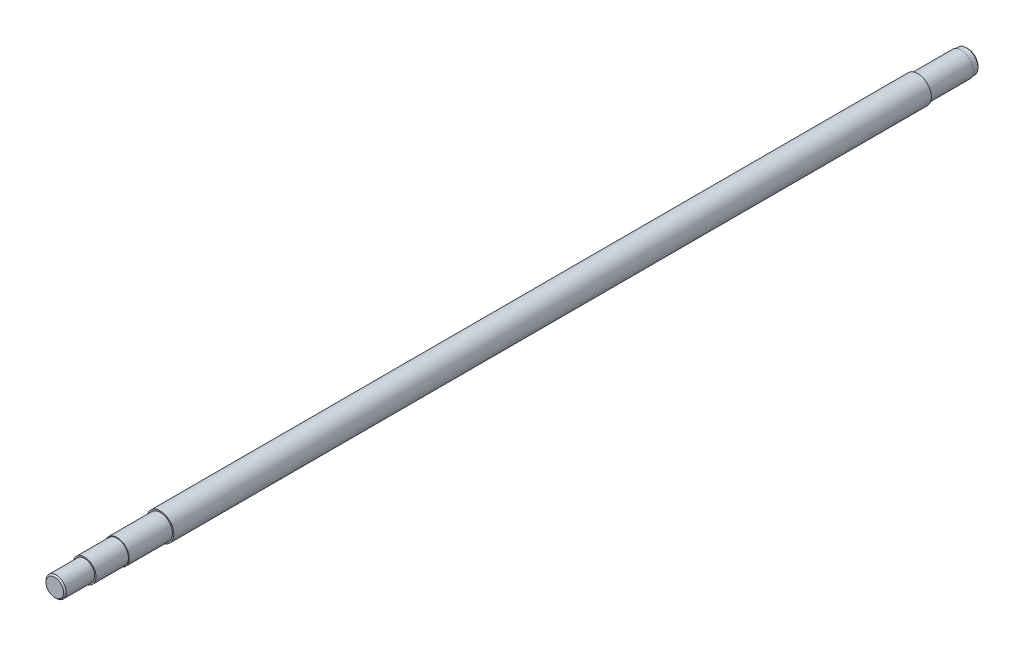
SolidWorks part; units mm, degrees
ref_plane "前视基准面" through (0, 0, 0) normal (0, 0, 1) x (1, 0, 0)
ref_plane "上视基准面" through (0, 0, 0) normal (0, 1, 0) x (1, 0, 0)
ref_plane "右视基准面" through (0, 0, 0) normal (1, 0, 0) x (0, 0, -1)
other "Configuration Table"
sketch "草图1" plane through (0, 0, 0) normal (0, 0, 1) x (1, 0, 0)
  circle A0 centre (0, 0) radius 37.5
  dimension "D1" = 75
extrude "凸台-拉伸1" add sketch "草图1" along normal blind 140 contours A0
sketch "草图2" plane through (0, 0, 140) normal (0, 0, 1) x (1, 0, 0)
  circle A0 centre (0, 0) radius 42.5
  dimension "D1" = 85
extrude "凸台-拉伸2" add sketch "草图2" along normal blind 120 contours A0
sketch "草图3" plane through (0, 0, 260) normal (0, 0, 1) x (1, 0, 0)
  circle A0 centre (0, 0) radius 45
  dimension "D1" = 90
extrude "凸台-拉伸3" add sketch "草图3" along normal blind 160 contours A0
sketch "草图4" plane through (0, 0, 420) normal (0, 0, 1) x (1, 0, 0)
  circle A0 centre (0, 0) radius 50
  dimension "D1" = 100
extrude "凸台-拉伸4" add sketch "草图4" along normal blind 2800 contours A0
sketch "草图5" plane through (0, 0, 3220) normal (0, 0, 1) x (1, 0, 0)
  circle A0 centre (0, 0) radius 45
  dimension "D1" = 90
extrude "凸台-拉伸5" add sketch "草图5" along normal blind 160 contours A0
sketch "草图6" plane through (0, 0, 3380) normal (0, 0, 1) x (1, 0, 0)
  circle A0 centre (0, 0) radius 42.5
  dimension "D1" = 85
extrude "凸台-拉伸6" add sketch "草图6" along normal blind 120 contours A0
sketch "草图7" plane through (0, 0, 3500) normal (0, 0, 1) x (1, 0, 0)
  circle A0 centre (0, 0) radius 37.5
  dimension "D1" = 75
extrude "凸台-拉伸7" add sketch "草图7" along normal blind 110 contours A0
sketch "草图8" plane through (0, 0, 0) normal (0, 0, -1) x (-1, 0, 0)
  circle A0 centre (0, 0) radius 75
  dimension "D1" = 150
extrude "切除-拉伸1" cut sketch "草图8" against normal blind 235 contours A0
chamfer "倒角1" distance 5 angle 45 2 edges at (-42.5, 0, 235) (37.5, 0, 3610)
